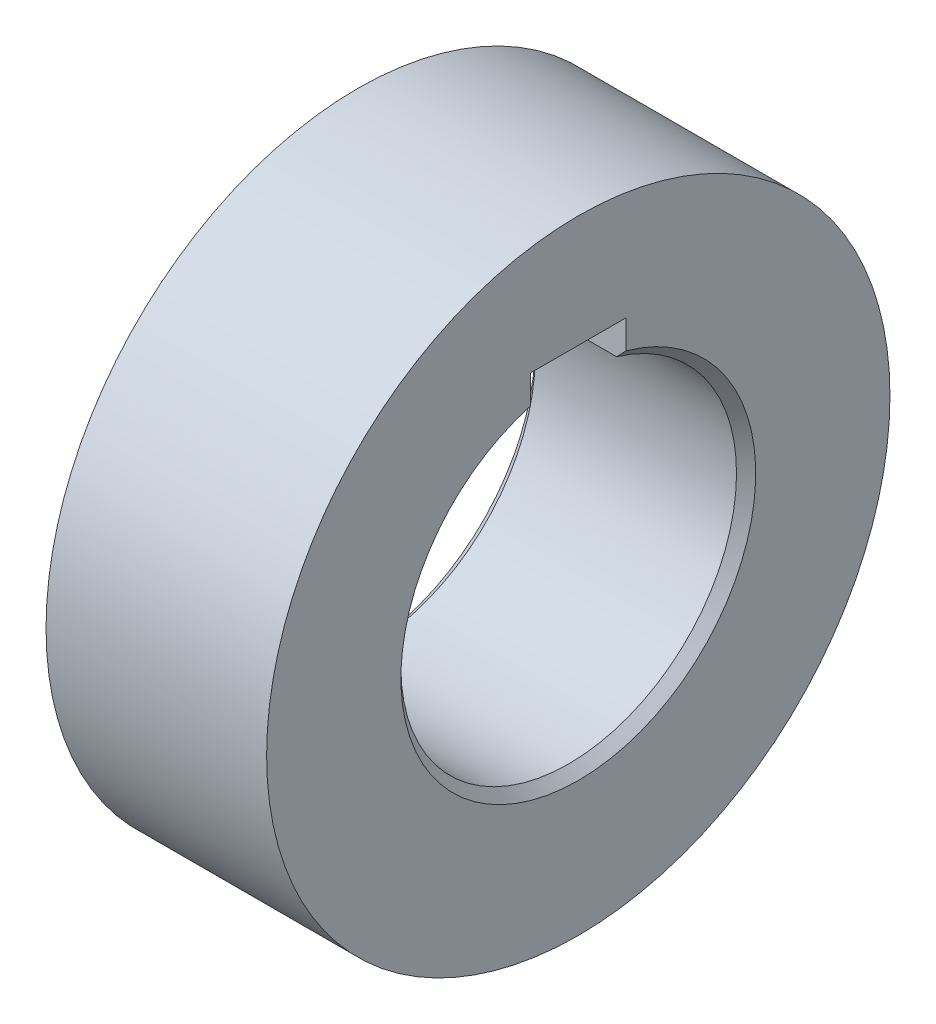
from build123d import *

# Parameters (mm, degrees)
CHAMFER_1_SIZE           = 1
SKETCH_4_W               = 10
SKETCH_4_H               = 4.029490121
CUT_EXTRUDE_1_DEPTH      = 69.000919111
CUT_EXTRUDE_3_DEPTH      = 23
CUT_EXTRUDE_3_DEPTH_BACK = 2
SKETCH_6_OUTSIDE_W       = 118.508
SKETCH_6_OUTSIDE_H       = 118.508
SKETCH_6_OUTSIDE_R       = 31.5
SKETCH_9_R               = 32.5
SKETCH_9_R_2             = 31.5
EXTRUDE_1_DEPTH          = 23


with BuildPart() as part:
    # 草图1 → 旋转1 (revolve)
    with BuildSketch(Plane.XY, mode=Mode.PRIVATE) as revolve_1_sk:
        Polygon((0, 17.5), (0, 45.25), (18, 45.25), (18, 31.5), (23, 31.5), (23, 17.5), align=None)
    revolve(revolve_1_sk.sketch.rotate(Axis((0, 0, 0), (1, 0, 0)), 90), axis=Axis((0, 0, 0), (1, 0, 0)))

    # 草图2 → 切除-旋转1 (revolve, cut)
    with BuildSketch(Plane.XY, mode=Mode.PRIVATE) as cut_revolve_1_sk:
        Polygon((11.840143071, 33.8), (15.340759374, 45.25), (2.659240626, 45.25), (6.159856929, 33.8), align=None)
    revolve(cut_revolve_1_sk.sketch.rotate(Axis((0, 0, 0), (1, 0, 0)), 90), axis=Axis((0, 0, 0), (1, 0, 0)), mode=Mode.SUBTRACT)

    # 倒角1
    chamfer_1_edges = [part.edges().sort_by_distance(p)[0] for p in [
        (0, 0, -17.5),
        (23, 0, -17.5),
    ]]
    chamfer(chamfer_1_edges, length=CHAMFER_1_SIZE)

    # 草图4 → 切除-拉伸1 (cut, through all)
    with BuildSketch(Plane.ZY):
        with Locations((0, 18.785254892)):
            Rectangle(SKETCH_4_W, SKETCH_4_H)
    extrude(amount=-CUT_EXTRUDE_1_DEPTH, mode=Mode.SUBTRACT)

    # 草图6 outside → 切除-拉伸3 (cut, two sides: drawn at the far end of the back side and taken through both)
    with BuildSketch(Plane(origin=(0, 0, 0), x_dir=(0, 0, -1), z_dir=(1, 0, 0)).offset(-CUT_EXTRUDE_3_DEPTH_BACK)):
        Rectangle(SKETCH_6_OUTSIDE_W, SKETCH_6_OUTSIDE_H)
        with Locations(Location((0, 0, 0), (0, 0, 180))):
            Circle(SKETCH_6_OUTSIDE_R, mode=Mode.SUBTRACT)
    extrude(amount=CUT_EXTRUDE_3_DEPTH + CUT_EXTRUDE_3_DEPTH_BACK, mode=Mode.SUBTRACT)

    # 草图9 → 凸台-拉伸1 (add)
    with BuildSketch(Plane(origin=(0, 0, 0), x_dir=(0, 0, -1), z_dir=(1, 0, 0))):
        Circle(SKETCH_9_R)
        Circle(SKETCH_9_R_2, mode=Mode.SUBTRACT)
    extrude(amount=EXTRUDE_1_DEPTH)


solid = part.part
